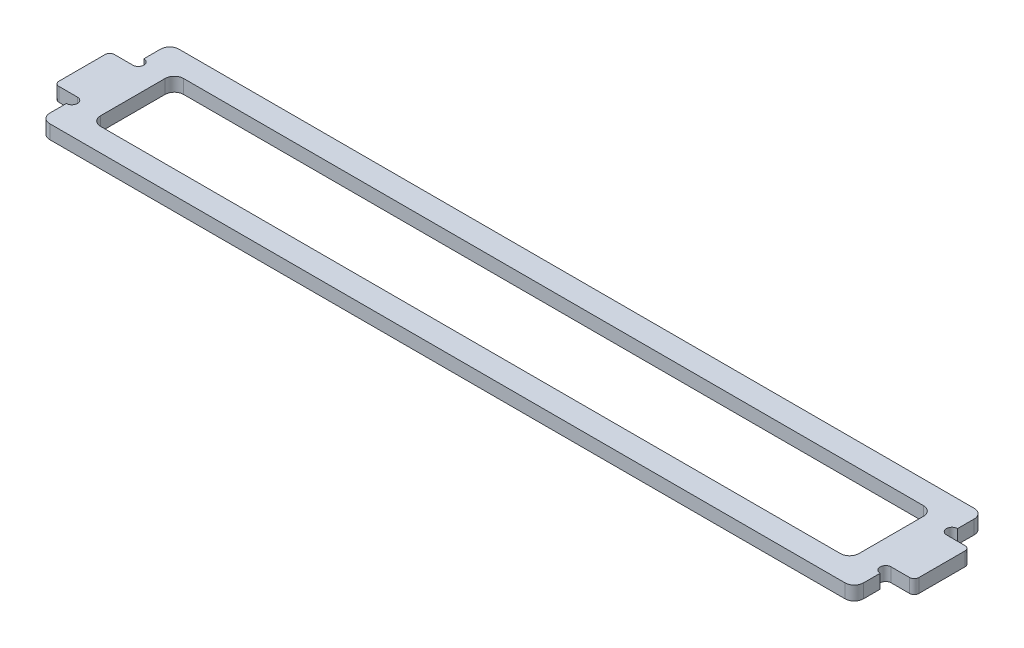
SolidWorks part; units mm, degrees
material "Thornel Mat VMA"
ref_plane "前视基准面" through (0, 0, 0) normal (0, 0, 1) x (1, 0, 0)
ref_plane "上视基准面" through (0, 0, 0) normal (0, 1, 0) x (1, 0, 0)
ref_plane "右视基准面" through (0, 0, 0) normal (1, 0, 0) x (0, 0, -1)
other "Configuration Table"
sketch "草图1" plane through (0, 0, 0) normal (0, 1, 0) x (1, 0, 0)
  line L0 (0, 0) -> (49.0116, 0) construction
  line L1 (-44.1, 7) -> (44.1, 7)
  line L2 (-44.1, 7) -> (-44.1, -7)
  line L3 (-44.1, -7) -> (44.1, -7)
  line L4 (44.1, 7) -> (44.1, -7)
  line L5 (-44.1, 7) -> (44.1, -7) construction
  line L6 (-44.1, -7) -> (44.1, 7) construction
  line L7 (0, 0) -> (0, 20.3889) construction
  line L8 (-44.1, 3) -> (-46.6, 3)
  line L9 (44.1, 3) -> (46.6, 3)
  line L10 (44.1, 3) -> (44.1, -3)
  line L11 (44.1, -3) -> (46.6, -3)
  line L12 (46.6, 3) -> (46.6, -3)
  line L13 (-46.6, 3) -> (-46.6, -3)
  line L14 (-44.1, -3) -> (-46.6, -3)
  line L16 (-41.1, 4.5) -> (41.1, 4.5)
  line L17 (-41.1, 4.5) -> (-41.1, -4.5)
  line L18 (-41.1, -4.5) -> (41.1, -4.5)
  line L19 (41.1, 4.5) -> (41.1, -4.5)
  line L20 (-41.1, 4.5) -> (41.1, -4.5) construction
  line L21 (-41.1, -4.5) -> (41.1, 4.5) construction
  circle A0 centre (44.1, 3.6) radius 0.6
  circle A1 centre (44.1, -3.6) radius 0.6
  circle A2 centre (-44.1, -3.6) radius 0.6
  circle A3 centre (-44.1, 3.6) radius 0.6
  point P0 (0, 0)
  dimension "D5" = 1.2
  dimension "D1" = 6
  dimension "D2" = 88.2
  dimension "D3" = 2.5
  dimension "D4" = 4
  dimension "D6" = 2.5
  dimension "D7" = 3
extrude "凸台-拉伸1" add sketch "草图1" along normal blind 1.5 contours L2 A3 A2 L3 L4 A1 A0 L1 L16 L19 L18 L17 | L14 L2 L8 L13 | L12 L9 L4 L11
fillet "圆角1" radius 0.5 4 edges at (-46.6, 0.75, 3) (-46.6, 0.75, -3) (46.6, 0.75, 3) (46.6, 0.75, -3)
fillet "圆角2" radius 1 8 edges at (-41.1, 0.75, 4.5) (41.1, 0.75, 4.5) (41.1, 0.75, -4.5) (-41.1, 0.75, -4.5) (-44.1, 0.75, -7) (-44.1, 0.75, 7) (44.1, 0.75, 7) (44.1, 0.75, -7)
